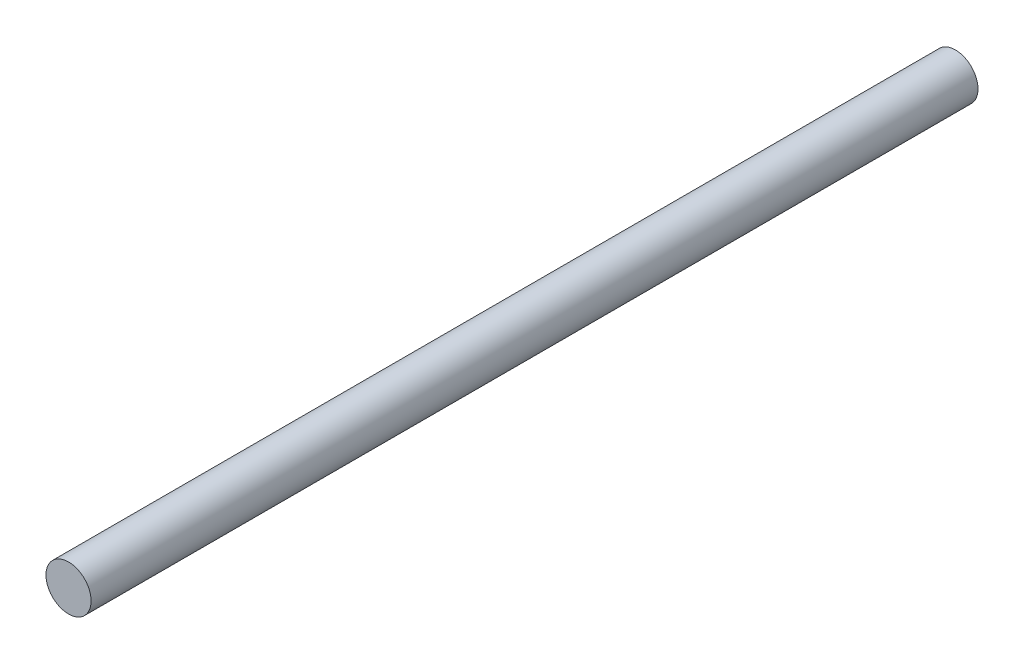
from build123d import *

# Parameters (mm, degrees)
SKETCH1_R           = 1.4
BOSS_EXTRUDE1_DEPTH = 27.5


with BuildPart() as part:
    # Sketch1 → Boss-Extrude1 (new, symmetric)
    with BuildSketch(Plane.XY):
        with Locations((-151.119026916, -87.731782697)):
            Circle(SKETCH1_R)
    extrude(amount=BOSS_EXTRUDE1_DEPTH, both=True)


solid = part.part
